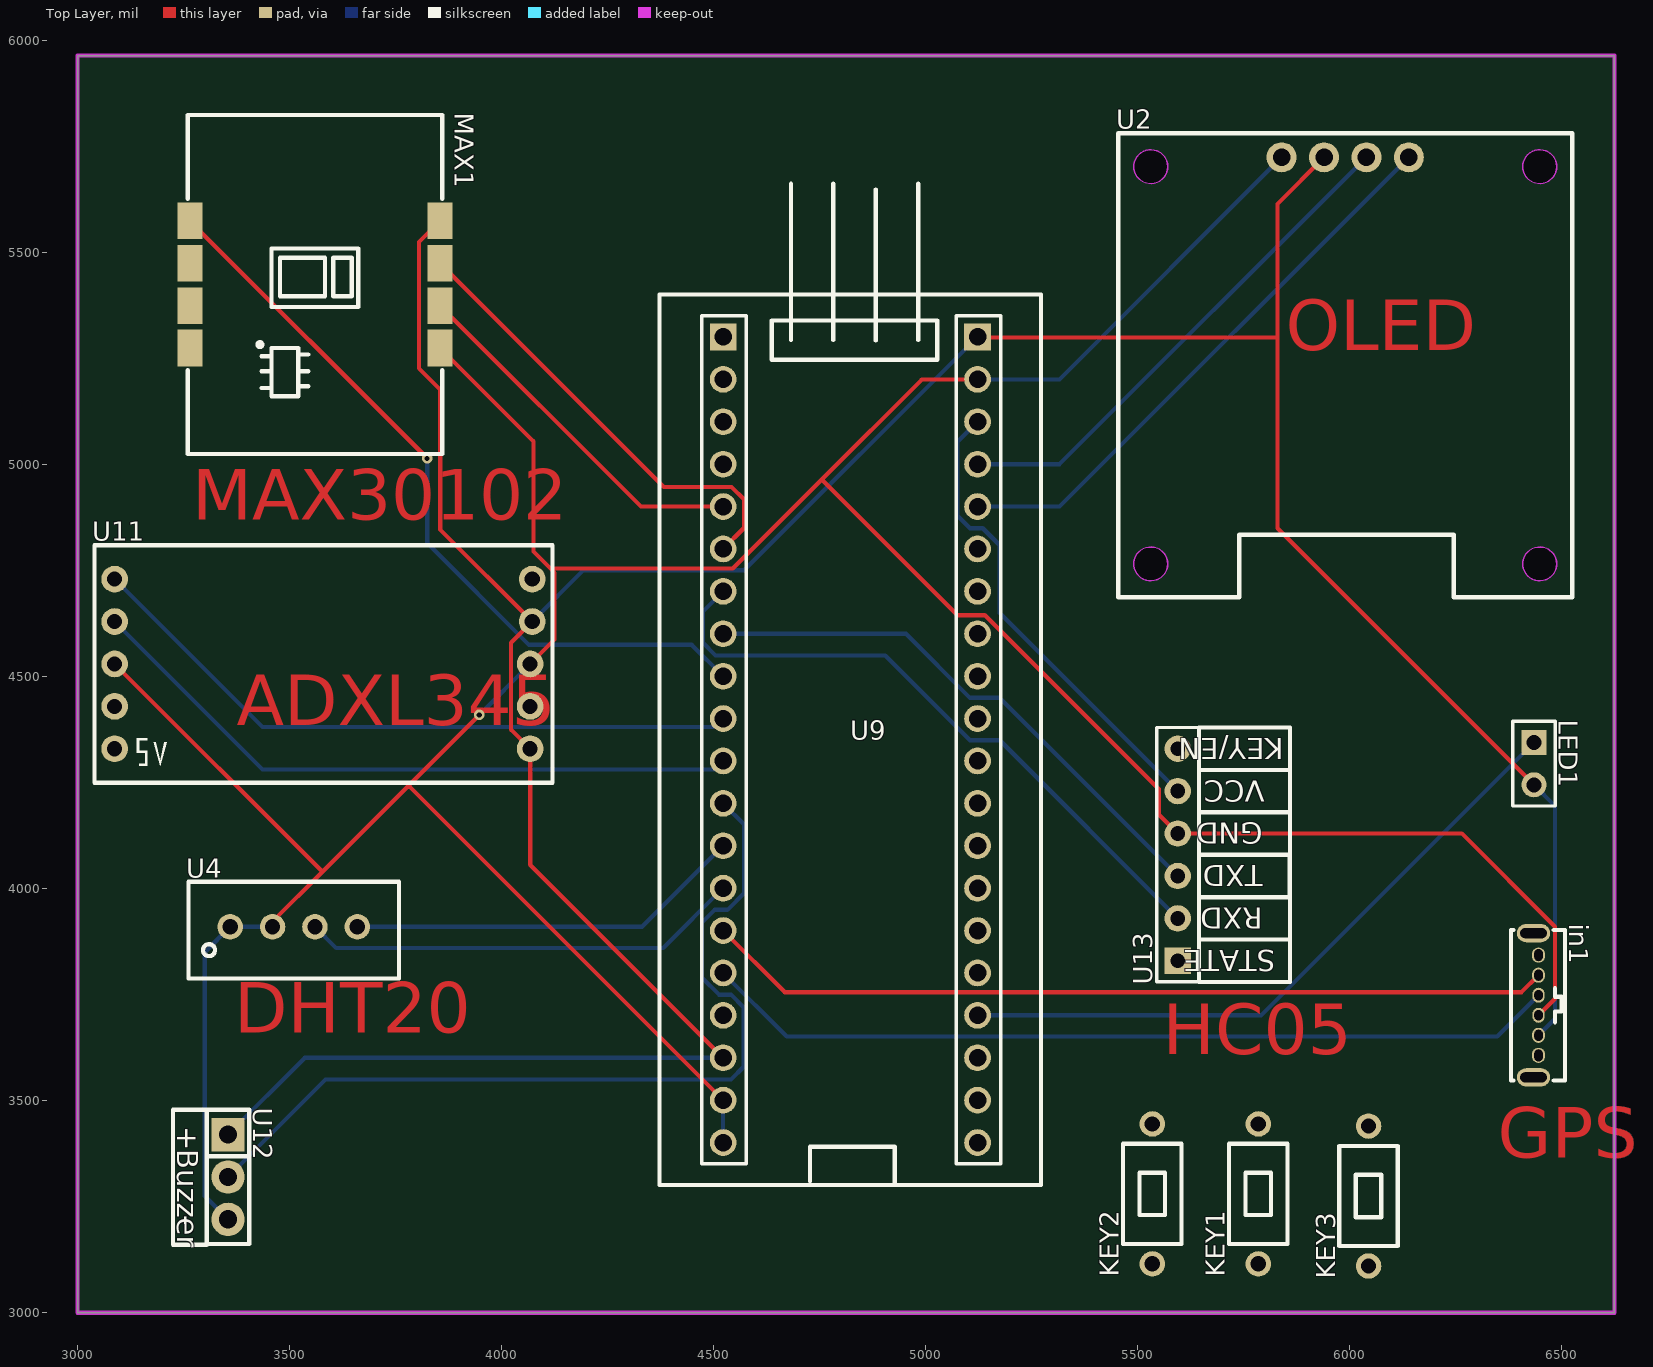
[diagram p0: Top Layer view]
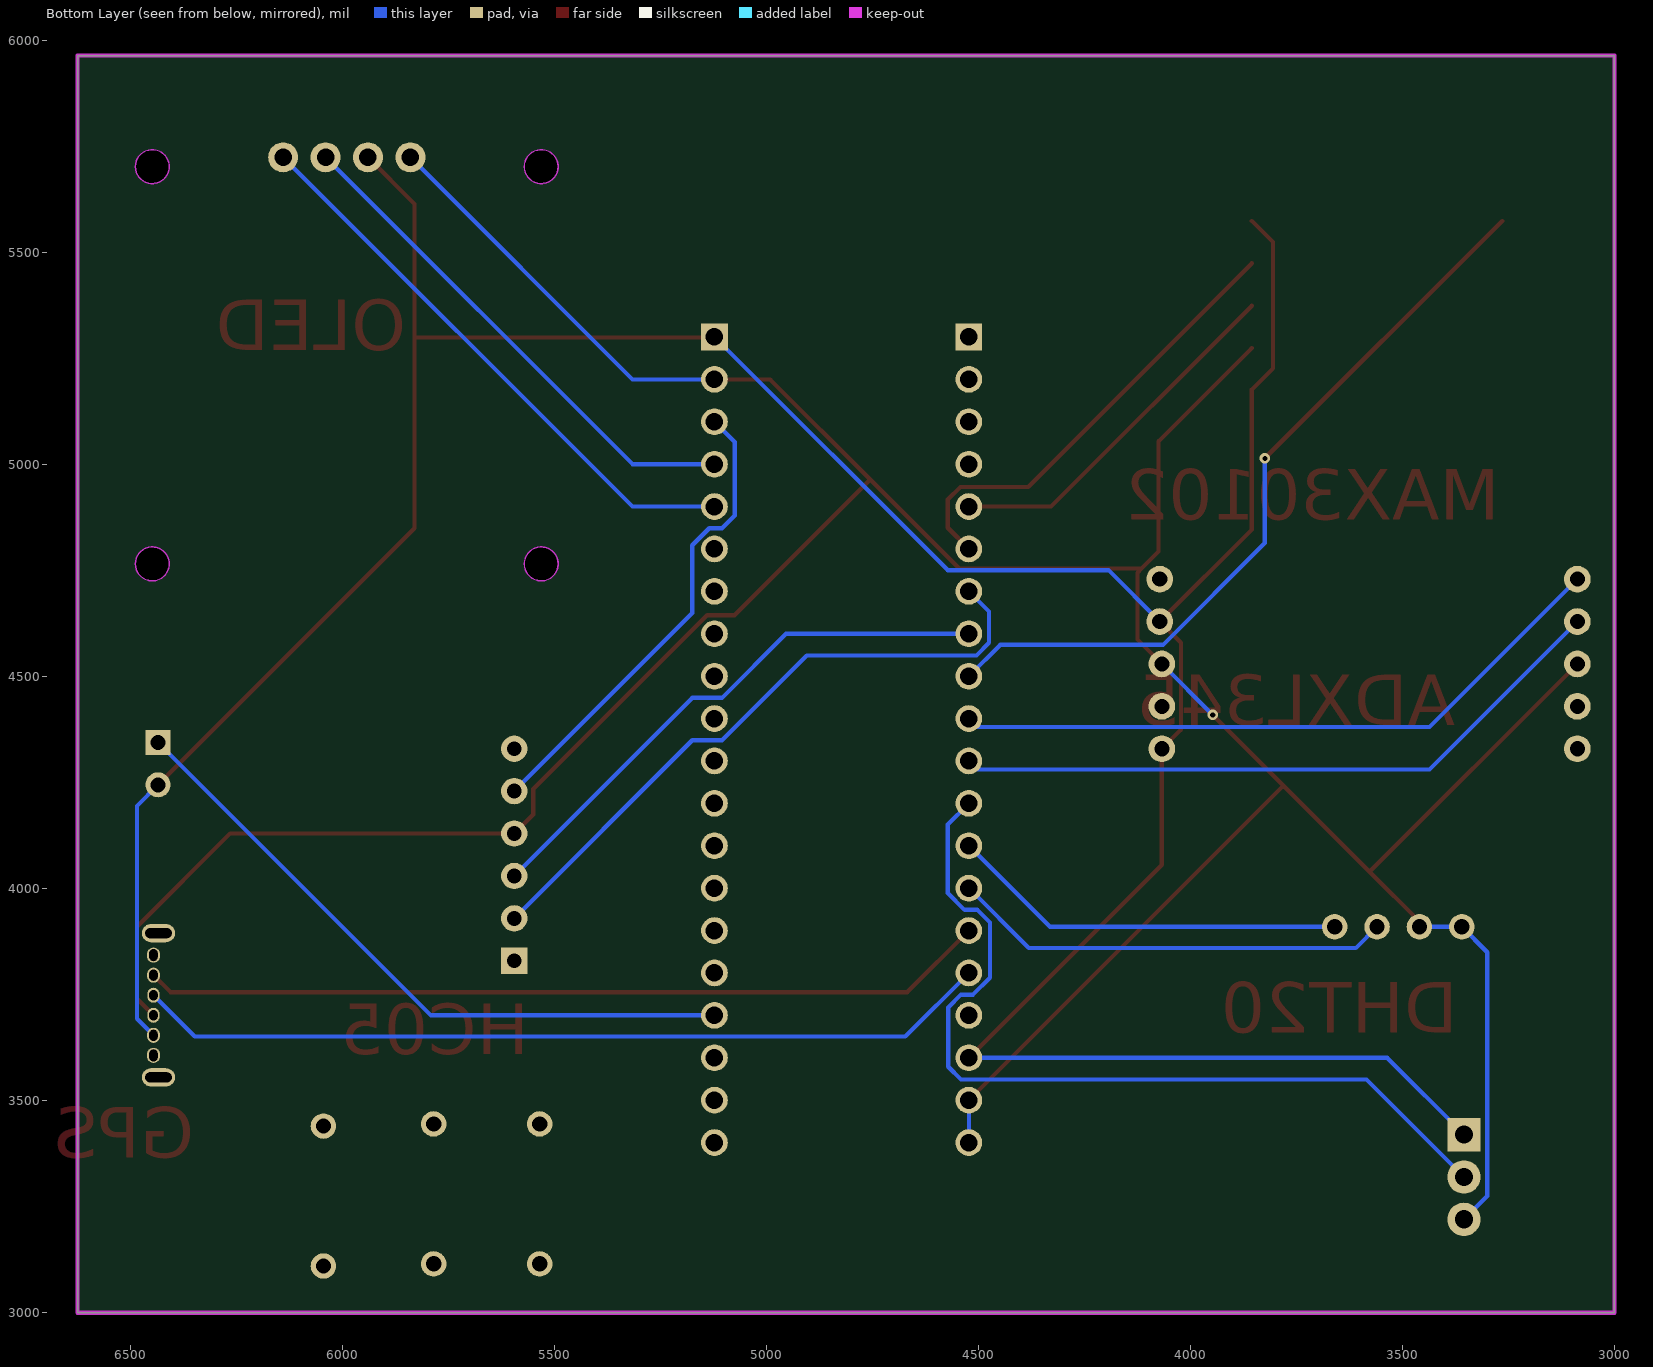
[diagram p1: Bottom Layer view, seen from below]
# Altium PCB MISC89051.pcbdoc
Units mil, origin at the board's own origin, x right, y up, seen from the top; angles counter-clockwise.
Board outline 3625 x 2965 mil, 2 copper layers (Top Layer, Bottom Layer), stack 62.206 mil thick; 12 components, 21 nets, 91 pads, 2 vias.

## Layer stack, top to bottom
Top Solder Mask Layer: solder mask 0.394, Dk 3.3
Top Layer: signal copper 1.379
Dielectric1: surface 59.449, FR4, Dk 4.5
Bottom Layer: signal copper 1.378
Bottom Solder Mask Layer: solder mask 0.394, Dk 3.3

## Board outline
3000,5965 3000,3000 6625,3000 6625,5965

## Design rules (kind name [scope] priority, off if disabled: settings)
BoardOutlineClearance copperThickness2oz_1 [All] p2 off: genericclearance=7.99 ignorepadtopadclearanceinfootprint=FALSE except(0: Arc-SplitContinuation Track-SplitContinuation SMDPad-SplitContinuation THPad-SplitContinuation Via-SplitContinuation Fill-SplitContinuation Region-SplitContinuation Poly-SplitContinuation Text-SplitContinuation Hole-SplitContinuation; 5.98: Arc-CutoutEdge SMDPad-CutoutEdge THPad-CutoutEdge Via-CutoutEdge Fill-CutoutEdge Region-CutoutEdge Text-CutoutEdge; 6.93: Hole-OutlineEdge Hole-CutoutEdge; 10: Poly-OutlineEdge Poly-CutoutEdge; 11.81: Arc-OutlineEdge Track-OutlineEdge SMDPad-OutlineEdge THPad-OutlineEdge Via-OutlineEdge Fill-OutlineEdge Region-OutlineEdge Text-OutlineEdge Track-CutoutEdge)
BoardOutlineClearance copperThickness1oz_1 [All] p4: genericclearance=4.02 ignorepadtopadclearanceinfootprint=FALSE except(0: Arc-SplitContinuation Track-SplitContinuation SMDPad-SplitContinuation THPad-SplitContinuation Via-SplitContinuation Fill-SplitContinuation Region-SplitContinuation Poly-SplitContinuation Text-SplitContinuation Hole-SplitContinuation; 6: SMDPad-CutoutEdge THPad-CutoutEdge Via-CutoutEdge Fill-CutoutEdge Region-CutoutEdge Text-CutoutEdge; 6.93: Hole-OutlineEdge Hole-CutoutEdge; 10: Poly-OutlineEdge Poly-CutoutEdge; 11.8: Arc-OutlineEdge Track-OutlineEdge SMDPad-OutlineEdge THPad-OutlineEdge Via-OutlineEdge Fill-OutlineEdge Region-OutlineEdge Text-OutlineEdge; 11.81: Arc-CutoutEdge Track-CutoutEdge)
Clearance copperThickness2oz [All] p1 off: gap=7.99 ignorepadtopadclearanceinfootprint=FALSE except(5.98: SMDPad-Track SMDPad-SMDPad THPad-Track SMDPad-THPad THPad-THPad Track-Via SMDPad-Via THPad-Via Via-Via Fill-Track Region-Track Fill-SMDPad Region-SMDPad Fill-THPad Region-THPad Fill-Via Region-Via Fill-Fill Fill-Region Region-Region Arc-Track Arc-SMDPad Arc-THPad Arc-Via Fill-Arc Region-Arc Arc-Arc Text-Track SMDPad-Text Text-THPad Text-Via Fill-Text Region-Text Arc-Text Text-Text; 6.93: Hole-Track Hole-SMDPad Hole-THPad Hole-Via Fill-Hole Region-Hole Hole-Arc Hole-Text; 10: Poly-Track Poly-SMDPad Poly-THPad Poly-Via Poly-Fill Poly-Region Poly-Poly Poly-Arc Poly-Text Poly-Hole)
Clearance copperThickness1oz [All] p3: gap=4.02 ignorepadtopadclearanceinfootprint=FALSE except(5.98: SMDPad-Track SMDPad-SMDPad THPad-Track SMDPad-THPad THPad-THPad Track-Via SMDPad-Via THPad-Via Via-Via Fill-Track Region-Track Fill-SMDPad Region-SMDPad Fill-THPad Region-THPad Fill-Via Region-Via Fill-Fill Fill-Region Region-Region; 6: Arc-Track Arc-SMDPad Arc-THPad Arc-Via Fill-Arc Region-Arc Arc-Arc Text-Track SMDPad-Text Text-THPad Text-Via Fill-Text Region-Text Arc-Text Text-Text; 6.93: Hole-Track Hole-SMDPad Hole-THPad Hole-Via Fill-Hole Region-Hole Hole-Arc Hole-Text; 10: Poly-Track Poly-SMDPad Poly-THPad Poly-Via Poly-Fill Poly-Region Poly-Poly Poly-Arc Poly-Text Poly-Hole)
DiffPairsRouting differentialPair [All] p1: maxlimit=6 minlimit=6 mostfreqgap=6 toplayer_minwidth=5 toplayer_prefwidth=10 toplayer_maxwidth=100 toplayer_mingap=6 toplayer_prefgap=6 toplayer_maxgap=6 bottomlayer_minwidth=5 bottomlayer_prefwidth=10 bottomlayer_maxwidth=100 bottomlayer_mingap=6 bottomlayer_prefgap=6 bottomlayer_maxgap=6 maxuncoupledlength=10
HoleToHoleClearance otherClearance [All] p1: gap=11.81 allowstackedmicrovias=TRUE
Length netLength [All] p1: minlimit=0 maxlimit=0
MatchedLengths netLengthTolerance [All] p1: tolerance=1000
PasteMaskExpansion pasteMaskExpansion [All] p1: expansion=0
PlaneConnect innerPlane [All] p1: planeconnectstyle=Relief reliefexpansion=20 reliefentries=4 reliefconductorwidth=10 reliefairgap=10
PolygonConnect copperRegion [All] p1: connectstyle=Relief reliefconductorwidth=10 reliefentries=4 polygonreliefangle="90 Angle" airgapwidth=10 via.connectstyle=Relief via.reliefconductorwidth=10 via.reliefentries=4 via.polygonreliefangle="90 Angle" via.airgapwidth=10
RoutingVias viaSize [All] p1: holewidth=12.01 width=24.02 viastyle="Through Hole" minholewidth=11.81 minwidth=19.68 maxholewidth=248.03 maxwidth=393.7
SolderMaskExpansion solderMaskExpansion [IsVia] p1: expansion=-1000 istentingtop=TRUE
SolderMaskExpansion solderMaskExpansion [All] p2: expansion=2 istentingtop=FALSE
Width copperThickness2oz_2 [All] p1 off: maxlimit=100 minlimit=8 preferedwidth=10
Width copperThickness1oz_2 [All] p2: maxlimit=100 minlimit=5 preferedwidth=10

## Components (designator, comment, footprint, x,y, rotation, side; value= is the part's Value field where it differs from the comment)
in1 "gps" TYPE-C-6PIN-TH_C9900014686 6440,3725 r270 top
KEY1 "Through-hole tact switch" 直插轻触开关3*6*5 5785,3120 r90 top
KEY2 "Through-hole tact switch" 直插轻触开关3*6*5 5535,3120 r90 top
KEY3 "Through-hole tact switch" 直插轻触开关3*6*5 6045,3115 r90 top
LED1 "LED" HDR1X2 6435,4345 r270 top
MAX1 "MAX30102 module" COMM-SMD_8P-L20.2-W15.4-P2.54_MAX30102 3560,5425 r270 top
U2 "0.96OLED" OLED-TH_L27.8-W27.2-P2.54_C9900033791 5990,5725 r0 top
U4 "DHT20" SENSOR-TH_DHT20 3510,3910 r0 top
U9 "STM32F103C8T6 minimum system board" STM32F103C8T6核心板 4822.68,4351.18 r0 top
U11 "ADXL345" COMM-TH_ADXL345 3580,4530 r0 top
U12 "Buzzer" 蜂鸣器 3355,3320 r270 top
U13 "HC-05" HC05_6P 5595,4030 r90 top

## Footprints (in the part's own frame and the unit in brackets; to place one, negate y for a bottom-side part, rotate by r counter-clockwise, add the part's x,y. Pads: shape width x height; smd on the part's side, far side on the other; paste and mask are expansions set on the pad)
COMM-SMD_8P-L20.2-W15.4-P2.54_MAX30102 [mm]
  rect 2.2x1.5 smd: 1(-3.81,-7.5) 2(-1.27,-7.5) 3(1.27,-7.5) 4(3.81,-7.5) 5(3.81,7.5) 6(1.27,7.5) 7(-1.27,7.5) 8(-3.81,7.5)
  silkscreen extent -10.16,-7.62 10.16,7.62
COMM-TH_ADXL345 [mm]
  round 1.6 hole 0.9: 1(-12.51,5.08) 2(-12.51,2.54) 3(-12.51,0) 4(-12.51,-2.54) 5(-12.51,-5.08) 6(12.383,-5.08) 7(12.383,-2.54) 8(12.383,0) 9(12.51,2.54) 10(12.51,5.08)
  silkscreen extent -13.72,-7.11 13.72,7.11
HC05_6P [mil]
  rect 62x62 hole 35 paste+0 mask+2: 1(-200,0)
  round 62 hole 35 paste+0 mask+2: 2(-100,0) 3(0,0) 4(100,0) 5(200,0) 6(300,0)
  silkscreen extent -250,-265 350,50
HDR1X2 [mm]
  rect 1.5x1.5 hole 0.9: 1(0,0)
  round 1.5 hole 0.9: 2(2.54,0)
  silkscreen extent -1.27,-1.27 3.81,1.27
OLED-TH_L27.8-W27.2-P2.54_C9900033791 [mm]
  round 1.8 hole 1.05 paste+0 mask+0.05: 1(-3.81,0) 2(-1.27,0) 3(1.27,0) 4(3.81,0)
  Board Outline Layer circle w0.003: c-11.65,-0.56 r1.016
  Board Outline Layer circle w0.003: c11.65,-0.56 r1.016
  Board Outline Layer circle w0.003: c-11.65,-24.36 r1.016
  Board Outline Layer circle w0.003: c11.65,-24.36 r1.016
  Board Outline Layer region: -10.634,-0.56 -10.735,-1.001 -11.016,-1.354 -11.424,-1.551 -11.876,-1.551 -12.283,-1.354 -12.565,-1.001 -12.666,-0.56 -12.666,-0.56 -12.565,-0.119 -12.283,0.234 -11.876,0.431 -11.424,0.431 -11.016,0.234 -10.735,-0.119 -10.634,-0.56
  Board Outline Layer region: -10.634,-0.56 -10.643,-0.698 -10.672,-0.834 -10.718,-0.965 -10.782,-1.088 -10.862,-1.201 -10.956,-1.303 -11.064,-1.39 -11.183,-1.462 -11.31,-1.517 -11.443,-1.555 -11.581,-1.574 -11.719,-1.574 -11.857,-1.555 -11.99,-1.517 -12.117,-1.462 -12.236,-1.39 -12.343,-1.303 -12.438,-1.201 -12.518,-1.088 -12.582,-0.965 -12.628,-0.834 -12.656,-0.698 -12.666,-0.56 -12.656,-0.422 -12.628,-0.286 -12.582,-0.155 -12.518,-0.032 -12.438,0.081 -12.343,0.183 -12.236,0.27 -12.117,0.342 -11.99,0.397 -11.857,0.435 -11.719,0.454 -11.581,0.454 -11.443,0.435 -11.31,0.397 -11.183,0.342 -11.064,0.27 -10.956,0.183 -10.862,0.081 -10.782,-0.032 -10.718,-0.155 -10.672,-0.286 -10.643,-0.422
  Board Outline Layer region: 12.666,-0.56 12.565,-1.001 12.283,-1.354 11.876,-1.551 11.424,-1.551 11.017,-1.354 10.735,-1.001 10.634,-0.56 10.634,-0.56 10.735,-0.119 11.017,0.234 11.424,0.431 11.876,0.431 12.283,0.234 12.565,-0.119 12.666,-0.56
  Board Outline Layer region: 12.666,-0.56 12.657,-0.698 12.628,-0.834 12.582,-0.965 12.518,-1.088 12.438,-1.201 12.343,-1.303 12.236,-1.39 12.117,-1.462 11.99,-1.517 11.857,-1.555 11.719,-1.574 11.581,-1.574 11.443,-1.555 11.31,-1.517 11.183,-1.462 11.064,-1.39 10.957,-1.303 10.862,-1.201 10.782,-1.088 10.718,-0.965 10.672,-0.834 10.643,-0.698 10.634,-0.56 10.643,-0.422 10.672,-0.286 10.718,-0.155 10.782,-0.032 10.862,0.081 10.957,0.183 11.064,0.27 11.183,0.342 11.31,0.397 11.443,0.435 11.581,0.454 11.719,0.454 11.857,0.435 11.99,0.397 12.117,0.342 12.236,0.27 12.343,0.183 12.438,0.081 12.518,-0.032 12.582,-0.155 12.628,-0.286 12.657,-0.422
  Board Outline Layer region: -10.634,-24.36 -10.735,-24.801 -11.016,-25.154 -11.424,-25.35 -11.876,-25.35 -12.283,-25.154 -12.565,-24.801 -12.666,-24.36 -12.666,-24.36 -12.565,-23.919 -12.283,-23.566 -11.876,-23.369 -11.424,-23.369 -11.016,-23.566 -10.735,-23.919 -10.634,-24.36
  Board Outline Layer region: -10.634,-24.36 -10.643,-24.498 -10.672,-24.634 -10.718,-24.765 -10.782,-24.888 -10.862,-25.001 -10.956,-25.102 -11.064,-25.19 -11.183,-25.262 -11.31,-25.317 -11.443,-25.355 -11.581,-25.374 -11.719,-25.374 -11.857,-25.355 -11.99,-25.317 -12.117,-25.262 -12.236,-25.19 -12.343,-25.102 -12.438,-25.001 -12.518,-24.888 -12.582,-24.765 -12.628,-24.634 -12.656,-24.498 -12.666,-24.36 -12.656,-24.222 -12.628,-24.086 -12.582,-23.955 -12.518,-23.832 -12.438,-23.719 -12.343,-23.617 -12.236,-23.53 -12.117,-23.458 -11.99,-23.403 -11.857,-23.365 -11.719,-23.346 -11.581,-23.346 -11.443,-23.365 -11.31,-23.403 -11.183,-23.458 -11.064,-23.53 -10.956,-23.617 -10.862,-23.719 -10.782,-23.832 -10.718,-23.955 -10.672,-24.086 -10.643,-24.222
  Board Outline Layer region: 12.666,-24.36 12.565,-24.801 12.283,-25.154 11.876,-25.35 11.424,-25.35 11.017,-25.154 10.735,-24.801 10.634,-24.36 10.634,-24.36 10.735,-23.919 11.017,-23.566 11.424,-23.369 11.876,-23.369 12.283,-23.566 12.565,-23.919 12.666,-24.36
  Board Outline Layer region: 12.666,-24.36 12.657,-24.498 12.628,-24.634 12.582,-24.765 12.518,-24.888 12.438,-25.001 12.343,-25.102 12.236,-25.19 12.117,-25.262 11.99,-25.317 11.857,-25.355 11.719,-25.374 11.581,-25.374 11.443,-25.355 11.31,-25.317 11.183,-25.262 11.064,-25.19 10.957,-25.102 10.862,-25.001 10.782,-24.888 10.718,-24.765 10.672,-24.634 10.643,-24.498 10.634,-24.36 10.643,-24.222 10.672,-24.086 10.718,-23.955 10.782,-23.832 10.862,-23.719 10.957,-23.617 11.064,-23.53 11.183,-23.458 11.31,-23.403 11.443,-23.365 11.581,-23.346 11.719,-23.346 11.857,-23.365 11.99,-23.403 12.117,-23.458 12.236,-23.53 12.343,-23.617 12.438,-23.719 12.518,-23.832 12.582,-23.955 12.628,-24.086 12.657,-24.222
  Multi-Layer board cut-out: -10.634,-0.56 -10.735,-1.001 -11.016,-1.354 -11.424,-1.551 -11.876,-1.551 -12.283,-1.354 -12.565,-1.001 -12.666,-0.56 -12.666,-0.56 -12.565,-0.119 -12.283,0.234 -11.876,0.431 -11.424,0.431 -11.016,0.234 -10.735,-0.119 -10.634,-0.56
  Multi-Layer board cut-out: 12.666,-0.56 12.565,-1.001 12.283,-1.354 11.876,-1.551 11.424,-1.551 11.017,-1.354 10.735,-1.001 10.634,-0.56 10.634,-0.56 10.735,-0.119 11.017,0.234 11.424,0.431 11.876,0.431 12.283,0.234 12.565,-0.119 12.666,-0.56
  Multi-Layer board cut-out: -10.634,-24.36 -10.735,-24.801 -11.016,-25.154 -11.424,-25.35 -11.876,-25.35 -12.283,-25.154 -12.565,-24.801 -12.666,-24.36 -12.666,-24.36 -12.565,-23.919 -12.283,-23.566 -11.876,-23.369 -11.424,-23.369 -11.016,-23.566 -10.735,-23.919 -10.634,-24.36
  Multi-Layer board cut-out: 12.666,-24.36 12.565,-24.801 12.283,-25.154 11.876,-25.35 11.424,-25.35 11.017,-25.154 10.735,-24.801 10.634,-24.36 10.634,-24.36 10.735,-23.919 11.017,-23.566 11.424,-23.369 11.876,-23.369 12.283,-23.566 12.565,-23.919 12.666,-24.36
  silkscreen extent -13.6,-26.36 13.6,1.44
SENSOR-TH_DHT20 [mil]
  round 60 hole 36: 1(-150,0) 2(-50,0) 3(50,0) 4(150,0)
  silkscreen extent -248,-122 248,106
STM32F103C8T6核心板 [mil]
  rect 63x63 hole 41.3 paste+4 mask+4: 1(-300,950) 40(300,950)
  round 63 hole 41.3 paste+4 mask+4: 2(-300,850) 3(-300,750) 4(-300,650) 5(-300,550) 6(-300,450) 7(-300,350) 8(-300,250) 9(-300,150) 10(-300,50) 11(-300,-50) 12(-300,-150) 13(-300,-250) 14(-300,-350) 15(-300,-450) 16(-300,-550) 17(-300,-650) 18(-300,-750) 19(-300,-850) 20(-300,-950) 21(300,-950) 22(300,-850) 23(300,-750) 24(300,-650) 25(300,-550) 26(300,-450) 27(300,-350) 28(300,-250) 29(300,-150) 30(300,-50) 31(300,50) 32(300,150) 33(300,250) 34(300,350) 35(300,450) 36(300,550) 37(300,650) 38(300,750) 39(300,850)
  silkscreen extent -450,-1050 450,1312
TYPE-C-6PIN-TH_C9900014686 [mm]
  oval 0.9x0.8 hole 0.5 slot 0.7 at 0 deg: 1(-3,0.15) 6(3,0.15)
  oval 0.9x0.76 hole 0.5 slot 0.65 at 0 deg: 2(-1.8,0.15) 5(1.8,0.15)
  oval 0.9x0.72 hole 0.5 slot 0.6 at 0 deg: 3(-0.6,0.15) 4(0.6,0.15)
  oval 1.1x2 hole 0.6 slot 1.6 at 90 deg copper offset 0,0: 7(4.32,-0.15) 8(-4.32,-0.15)
  silkscreen extent -4.5,-1.5 4.5,1.73
直插轻触开关3*6*5 [mil]
  round 60 hole 36 paste+0 mask+2: 1(-5,0) 2(325,0)
  silkscreen extent 42,-69 278,69
蜂鸣器 [mm]
  rect 2x2 hole 1.1 paste+0 mask+0.051: 1(-2.54,0)
  round 2 hole 1.1 paste+0 mask+0.051: 2(0,0) 3(2.54,0)
  silkscreen extent -4.02,-3.3 4.06,1.27

## Via types
v1: diameter 24.02, hole 12, Top Layer to Bottom Layer, 2 vias

## Nets (pads, with @x,y where several pads share a name; then routed paths per layer and width w, separated by ;. In a path a pad name is that pad's centre, name@x,y a point inside that pad or via, vN(x,y) a via of type N, cw(c..) or ccw(c..) an arc to the next point about the centre after c; other vN are vias at no path point)
+5V: U9.38 U13.5 | length 1123.9
  Bottom Layer w10: U9.38 5075,5053.5 5075,4880 5105,4850 5135,4850 5175,4810 5175,4650 U13.5
GND: in1.4 MAX1.5 U2.1 U4.1 U4.2 U9.19 U9.20 U9.39 U11.3 U11.8 U12.3 U13.4 | length 8987.4
  Top Layer w10: U11.3 3577.5,4040 ; U4.2 3460,3922.5 3577.5,4040 ; MAX1.5 4075.27,5055 4075.27,4795 4115.27,4755 ; v1(3947.5,4410) 3777.5,4240 ; U11.8 4125.27,4587.77 4125.27,4745 4115.27,4755 ; U9.19 3783.86,4240 3777.5,4240 ; U9.39 4991.44,5201.17 4755.27,4965 ; in1.4 6485,3740.47 6485,3910 6265,4130 U13.4 5549.99,4175 5549.99,4235 5140,4645 5075.27,4645 4755.27,4965 ; 3577.5,4040 3777.5,4240 ; 4115.27,4755 4545.27,4755 4755.27,4965
  Bottom Layer w10: U12.3 3300,3275 3300,3850 U4.1 U4.2 ; v1(3947.5,4410) U11.8 ; U9.20 U9.19 ; U9.39 5316.18,5201.17 U2.1
PA0: MAX1.6 U9.5 | length 863.7
  Top Layer w10: MAX1.6 4329.1,4901.18 U9.5
PA1: MAX1.7 U9.6 | length 1085.4
  Top Layer w10: MAX1.7 4382.68,4947.6 4542.68,4947.6 4572.68,4917.6 4572.68,4851.18 U9.6
PA2: U9.7 U13.2 | length 1530.2
  Bottom Layer w10: U9.7 4475,4653.5 4475,4580 4505,4550 4905,4550 5105,4350 5175,4350 U13.2
PA3: U9.8 U13.3 | length 1308.9
  Bottom Layer w10: U9.8 4953.82,4601.18 5105,4450 5175,4450 U13.3
PA4: MAX1.1 U9.9 | length 1819.9
  Top Layer w10: MAX1.1 v1(3824.72,5015)
  Bottom Layer w10: v1(3824.72,5015) 3824.72,4815 4064.72,4575 4448.85,4575 U9.9
PA5: U9.10 U11.1 | length 1587.9
  Bottom Layer w10: U11.1 3436.32,4381.18 4502.68,4381.18 U9.10
PA6: U9.11 U11.2 | length 1587.9
  Bottom Layer w10: U11.2 3436.32,4281.18 4502.68,4281.18 U9.11
PA7: U9.12 U12.2 | length 2082.9
  Bottom Layer w10: U12.2 3585,3550 4541.5,3550 4571.5,3580 4571.5,3720 4541.5,3750 4512.68,3750 4472.68,3790 4472.68,3920 4502.68,3950 4532.68,3950 4572.68,3990 4572.68,4151.18 U9.12
PA8: U9.25
PA10: U9.27
PA12: U9.29
PB0: U4.4 U9.13 | length 941.9
  Bottom Layer w10: U4.4 4331.5,3910 U9.13
PB1: U4.3 U9.14 | length 1041.9
  Bottom Layer w10: U4.3 3610,3860 4381.5,3860 U9.14
PB8: U2.3 U9.37 | length 1217.1
  Bottom Layer w10: U9.37 5316.18,5001.18 U2.3
PB9: U2.4 U9.36 | length 1358.6
  Bottom Layer w10: U9.36 5316.18,4901.18 U2.4
PB10: in1.2 U9.15 | length 2000
  Top Layer w10: U9.15 4667.99,3755.87 6405.91,3755.87 in1.2
PB11: in1.3 U9.16 | length 2025.7
  Bottom Layer w10: U9.16 4672.68,3651.18 6348.46,3651.18 in1.3
PB15: LED1.1 U9.24 | length 1579
  Bottom Layer w10: U9.24 5791.18,3701.18 LED1.1
VCC: in1.5 LED1.2 MAX1.8 U2.2 U9.18 U9.40 U11.6 U11.9 U12.1 | length 8015.8
  Top Layer w10: MAX1.8 3805.27,5525 3805.27,5227.22 3855.27,5177.22 3855.27,4847.22 U11.9 4022.5,4580 4022.5,4375 U11.6 4067.5,4056.36 U9.18 ; U9.40 5123.85,5300 5830,5300 ; U2.2 5830,5615 5830,5300 ; LED1.2 5830,4850 5830,5300
  Bottom Layer w10: U12.1 3536.18,3601.18 U9.18 ; U11.9 4193.67,4751.18 4572.68,4751.18 U9.40 ; LED1.2 6485,4195 6485,3693.23 in1.5
pads on no net: in1.1 in1.6 in1.7 in1.8 KEY1.1 KEY1.2 KEY2.1 KEY2.2 KEY3.1 KEY3.2 MAX1.2 MAX1.3 MAX1.4 U9.1 U9.2 U9.3 U9.4 U9.17 U9.21 U9.22 U9.23 U9.26 U9.28 U9.30 U9.31 U9.32 U9.33 U9.34 U9.35 U11.4 U11.5 U11.7 U11.10 U13.1 U13.6

## Keep-outs
Board Outline Layer:
  the board outline again, w10

## Other copper
Top Layer:
  text "OLED" at 5850,5270 h120
  text "MAX30102" at 3270,4870 h120
  text "ADXL345" at 3375,4385 h120
  text "DHT20" at 3370,3660 h120
  text "HC05" at 5560,3610 h120
  text "GPS" at 6350,3365 h120